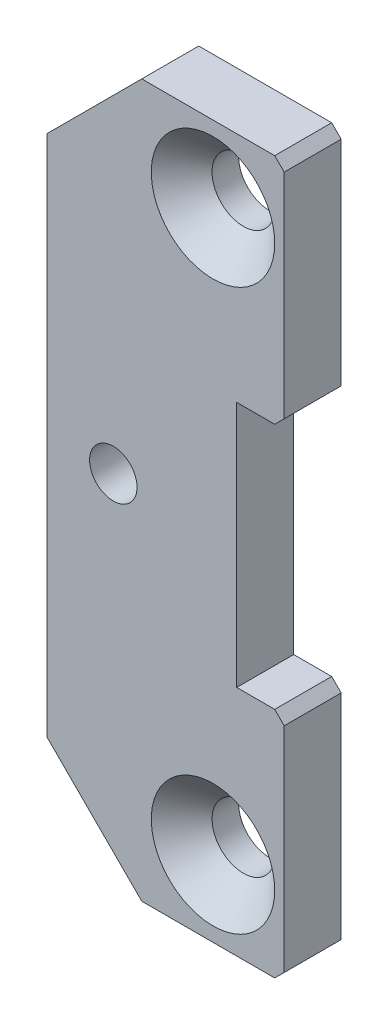
from build123d import *

# Parameters (mm, degrees)
SKETCH1_W                                   = 25
SKETCH1_H                                   = 75
EXTRUDE_THIN1_DEPTH                         = 6
CHAMFER1_SIZE                               = 1
HOLE_SIZE_PER_SOCKET_FLAT_COUNTEBLZ_2_COUNT = 2
HOLE_SIZE_PER_SOCKET_FLAT_COUNTEBLZ_2_PITCH = 59
CHAMFER2_SIZE                               = 10
M6_TAPPED_HOLE1_D                           = 5
SKETCH12_W                                  = 20.259222761
SKETCH12_H                                  = 26
CUT_EXTRUDE1_DEPTH                          = 10
CHAMFER3_SIZE                               = 1


with BuildPart() as part:
    # Sketch1 → Extrude-Thin1 (new body)
    with BuildSketch(Plane.XY):
        with Locations((-12.5, 37.5)):
            Rectangle(SKETCH1_W, SKETCH1_H)
    extrude(amount=EXTRUDE_THIN1_DEPTH)

    # Chamfer1
    chamfer1_edges = [part.edges().sort_by_distance(p)[0] for p in [
        (0, 75, 3),
        (0, 0, 3),
    ]]
    chamfer(chamfer1_edges, length=CHAMFER1_SIZE)

    # Sketch9 → Hole size (per socket flat counteBLZKk head screw type)1 (revolve, cut)
    with BuildSketch(Plane(origin=(-7.5, 67, 6), x_dir=(0, -1, 0), z_dir=(1, 0, 0))):
        Polygon((0, 0), (0, 6), (3.3, 6), (3.3, 3.2), (6.5, 0), align=None)
    hole_size_per_socket_flat_counteblzkk_h = revolve(axis=Axis((-7.5, 67, 12.35), (0, 0, -1)), mode=Mode.SUBTRACT)

    # Hole size _per socket flat counteBLZ 2: Hole size (per socket flat counteBLZKk head screw type)1 ×2
    with Locations(*[(0, -i * HOLE_SIZE_PER_SOCKET_FLAT_COUNTEBLZ_2_PITCH, 0) for i in range(1, HOLE_SIZE_PER_SOCKET_FLAT_COUNTEBLZ_2_COUNT)]):
        add(hole_size_per_socket_flat_counteblzkk_h, mode=Mode.SUBTRACT)

    # Chamfer2
    chamfer2_edges = [part.edges().sort_by_distance(p)[0] for p in [
        (-25, 75, 3),
        (-25, 0, 3),
    ]]
    chamfer(chamfer2_edges, length=CHAMFER2_SIZE)

    # M6 Tapped Hole1 (through all)
    with Locations(Plane.XY.offset(6)):
        with Locations((-18, 37.5)):
            Hole(M6_TAPPED_HOLE1_D / 2)

    # Sketch12 → Cut-Extrude1 (cut)
    with BuildSketch(Plane.XY.offset(6)):
        with Locations((5.129611381, 37.5)):
            Rectangle(SKETCH12_W, SKETCH12_H)
    extrude(amount=-CUT_EXTRUDE1_DEPTH, mode=Mode.SUBTRACT)

    # Chamfer3
    chamfer3_edges = [part.edges().sort_by_distance(p)[0] for p in [
        (0, 50.5, 3),
        (0, 24.5, 3),
    ]]
    chamfer(chamfer3_edges, length=CHAMFER3_SIZE)


solid = part.part
